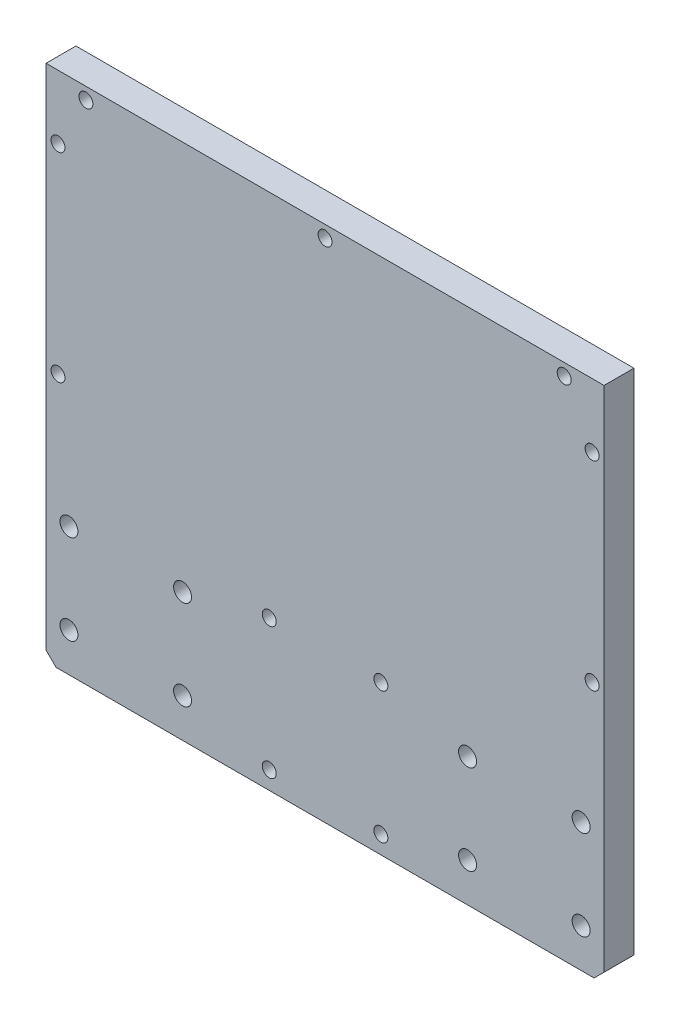
SolidWorks part; units mm, degrees
ref_plane "前视" through (0, 0, 0) normal (0, 0, 1) x (1, 0, 0)
ref_plane "上视" through (0, 0, 0) normal (0, 1, 0) x (1, 0, 0)
ref_plane "右视" through (0, 0, 0) normal (1, 0, 0) x (0, 0, -1)
sketch "草图1" plane through (0, 0, 0) normal (0, 0, 1) x (1, 0, 0)
  line L1 (0, 0) -> (280, 0)
  line L2 (0, 0) -> (0, -260)
  line L3 (0, -260) -> (280, -260)
  line L4 (280, 0) -> (280, -260)
  dimension "D1" = 280
  dimension "D2" = 260
extrude "凸台-拉伸1" add sketch "草图1" along normal blind 15
chamfer "倒角1" distance 5 angle 45 2 edges at (280, -260, 7.5) (0, -260, 7.5)
hole_wizard "Ø7.0 (7) 直径孔3" positions "草图3" profile "草图2" hole size "Ø7.0" standard "ISO" end condition through all
sketch "草图3" plane through (0, 0, 0) normal (0, 0, -1) x (-1, 0, 0)
  line L1 (-168, -185) -> (-112, -185)
  line L2 (-168, -185) -> (-168, -251)
  line L3 (-168, -251) -> (-112, -251)
  line L4 (-112, -185) -> (-112, -251)
  line L5 (-140, -251) -> (-140, -260) construction
  line L6 (-5, -260) -> (-275, -260) construction
  point P0 (-168, -185)
  point P3 (-112, -185)
  point P6 (-112, -251)
  point P9 (-168, -251)
  dimension "D1" = 56
  dimension "D2" = 66
  dimension "D3" = 9
sketch "草图2" plane through (168, -185, 0) normal (1, 0, 0) x (0, 1, 0)
  line L0 (0, 0) -> (0, 15)
  line L1 (0, 15) -> (3.5, 15)
  line L2 (3.5, 15) -> (3.5, 0)
  line L5 (3.5, 0) -> (0, 0)
  line L11 (0, -6.35) -> (0, 107.95) construction
  dimension "通孔孔直径" = 7
  dimension "通孔孔深度" = 15
hole_wizard "Ø7.0 (7) 直径孔2" positions "草图5" profile "草图4" hole size "Ø7.0" standard "ISO" end condition through all
sketch "草图5" plane through (0, 0, 15) normal (0, 0, 1) x (1, 0, 0)
  line L0 (20, -6) -> (140, -6) construction
  line L1 (140, -6) -> (260, -6) construction
  line L4 (140, -6) -> (140, 0) construction
  line L5 (280, 0) -> (0, 0) construction
  point P0 (20, -6)
  point P2 (260, -6)
  point P4 (140, -6)
  dimension "D1" = 6
  dimension "D2" = 120
sketch "草图4" plane through (20, -6, 15) normal (1, 0, 0) x (0, -1, 0)
  line L0 (0, 0) -> (0, 15)
  line L1 (0, 15) -> (3.5, 15)
  line L2 (3.5, 15) -> (3.5, 0)
  line L5 (3.5, 0) -> (0, 0)
  line L11 (0, -6.35) -> (0, 107.95) construction
  dimension "通孔孔直径" = 7
  dimension "通孔孔深度" = 15
hole_wizard "Ø9.0 (9) 直径孔1" positions "草图9" profile "草图8" hole size "Ø9.0" standard "ISO" end condition through all
sketch "草图9" plane through (0, 0, 0) normal (0, 0, -1) x (-1, 0, 0)
  line L0 (-140, -260) -> (-140, -2.5) construction
  line L1 (-5, -260) -> (-275, -260) construction
  line L3 (-268.5, -195.5) -> (-211.5, -195.5) construction
  line L4 (-211.5, -195.5) -> (-211.5, -240.5) construction
  line L5 (-211.5, -240.5) -> (-268.5, -240.5) construction
  line L6 (-268.5, -240.5) -> (-268.5, -195.5) construction
  circle A0 centre (-140, -6) radius 3.5 construction
  point P0 (-268.5, -240.5)
  point P3 (-268.5, -195.5)
  point P6 (-211.5, -195.5)
  point P9 (-211.5, -240.5)
  point P42 (-68.5, -240.5)
  point P43 (-68.5, -195.5)
  point P44 (-11.5, -195.5)
  point P45 (-11.5, -240.5)
  dimension "D1" = 19.5
  dimension "D2" = 71.5
  dimension "D3" = 57
  dimension "D4" = 45
sketch "草图8" plane through (268.5, -240.5, 0) normal (1, 0, 0) x (0, 1, 0)
  line L0 (0, 0) -> (0, 15)
  line L1 (0, 15) -> (4.5, 15)
  line L2 (4.5, 15) -> (4.5, 0)
  line L5 (4.5, 0) -> (0, 0)
  line L11 (0, -6.35) -> (0, 107.95) construction
  dimension "通孔孔直径" = 9
  dimension "通孔孔深度" = 15
hole_wizard "Ø7.0 (7) 直径孔1" positions "草图11" profile "草图10" hole size "Ø7.0" standard "ISO" end condition through all
sketch "草图11" plane through (0, 0, 15) normal (0, 0, 1) x (1, 0, 0)
  line L0 (274, -32) -> (274, -132) construction
  line L3 (6, -32) -> (6, -132) construction
  line L6 (274, -32) -> (274, 0) construction
  line L7 (280, 0) -> (0, 0) construction
  line L10 (6, -32) -> (6, 0) construction
  line L13 (0, 0) -> (0, -255) construction
  line L14 (280, -255) -> (280, 0) construction
  point P0 (6, -32)
  point P4 (274, -32)
  point P9 (274, -132)
  point P14 (6, -132)
  dimension "D1" = 6
  dimension "D2" = 6
  dimension "D3" = 100
  dimension "D4" = 32
sketch "草图10" plane through (6, -32, 15) normal (1, 0, 0) x (0, -1, 0)
  line L0 (0, 0) -> (0, 15)
  line L1 (0, 15) -> (3.5, 15)
  line L2 (3.5, 15) -> (3.5, 0)
  line L5 (3.5, 0) -> (0, 0)
  line L11 (0, -6.35) -> (0, 107.95) construction
  dimension "通孔孔直径" = 7
  dimension "通孔孔深度" = 15
